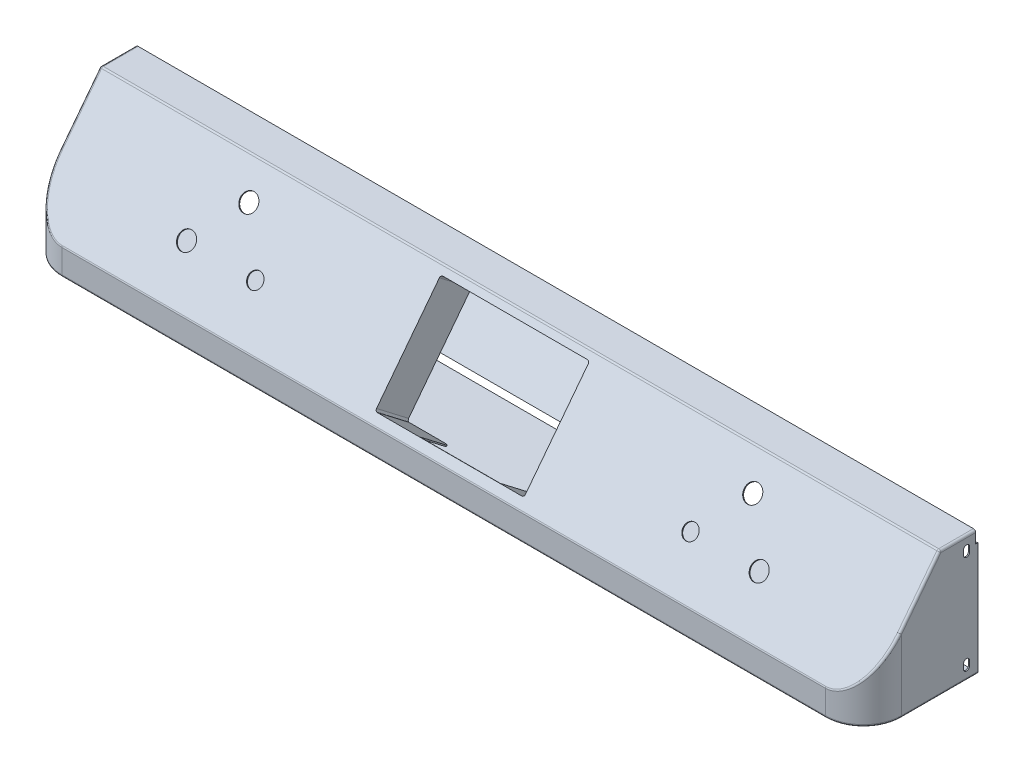
from build123d import *

# Parameters (mm, degrees)
SKETCH_1_W            = 1100
SKETCH_1_H            = 150
EXTRUDE_1_DEPTH       = 165
CUT_EXTRUDE_8_DEPTH   = 1115.831825882
FILLET_2_R            = 50
SHELL_1_T             = -1.5
HOLE_WIZARD_8_0_8_1_D = 8
SKETCH_20_W           = 83.034991693
SKETCH_20_H           = 41.985572191
CUT_EXTRUDE_7_DEPTH   = 1115.831825882
FILLET_5_R            = 3
CUT_EXTRUDE_10_DEPTH  = 1115.831825988
CUT_EXTRUDE_11_DEPTH  = 10
EXTRUDE_2_DEPTH       = 51.5
EXTRUDE_3_DEPTH       = 1.5
SKETCH_27_W           = 130
SKETCH_27_H           = 54.986401043
CUT_EXTRUDE_12_DEPTH  = 1.5
MOVE_FACE_1_BY        = 25
FILLET_6_R            = 10
SKETCH_28_R           = 11.25
SKETCH_28_R_2         = 9.75
CUT_EXTRUDE_13_DEPTH  = 1.5


with BuildPart() as part:
    # 草图1 → 凸台-拉伸1 (new body)
    with BuildSketch(Plane(origin=(0, 0, 0), x_dir=(1, 0, 0), z_dir=(0, 1, 0))):
        Rectangle(SKETCH_1_W, SKETCH_1_H)
    extrude(amount=EXTRUDE_1_DEPTH)

    # 草图21 → 切除-拉伸8 (cut, through all)
    with BuildSketch(Plane.ZY.offset(550)):
        Polygon((-25, 165), (75, 35), (149.01608628, 35), (149.01608628, 165), align=None)
    extrude(amount=-CUT_EXTRUDE_8_DEPTH, mode=Mode.SUBTRACT)

    # 圆角2
    fillet_2_edges = [part.edges().sort_by_distance(p)[0] for p in [
        (550, 17.5, 75),
        (-550, 17.5, 75),
    ]]
    fillet(fillet_2_edges, radius=FILLET_2_R)

    # 抽壳1
    shell_1_openings = [part.faces().sort_by_distance(p)[0] for p in [
        (0, 82.5, -75),
    ]]
    offset(amount=SHELL_1_T, openings=shell_1_openings, kind=Kind.INTERSECTION)

    # Ø8.0 (8) 直径孔1 (through all)
    with Locations(Plane.ZY.offset(550)):
        with Locations((-60, 147), (-60, 18)):
            Hole(HOLE_WIZARD_8_0_8_1_D / 2)

    # 草图20 → 切除-拉伸7 (cut, through all)
    with BuildSketch(Plane.ZY.offset(550)):
        with Locations((-113.517495847, 169.992786096)):
            Rectangle(SKETCH_20_W, SKETCH_20_H)
    extrude(amount=-CUT_EXTRUDE_7_DEPTH, mode=Mode.SUBTRACT)

    # 圆角5
    fillet_5_edges = [part.edges().sort_by_distance(p)[0] for p in [
        (550, 165, -48.5),
        (0, 165, -25),
        (-550, 132.5, 0),
        (550, 132.5, 0),
        (550, 0, -25),
        (0, 0, 75),
        (-535.355339059, 0, 60.355339059),
        (535.355339059, 0, 60.355339059),
        (0, 35, 75),
        (-539.140260323, 59.552655996, 56.113341541),
        (539.140260323, 59.552655996, 56.113341541),
        (-550, 0, -25),
        (-550, 165, -48.5),
    ]]
    fillet(fillet_5_edges, radius=FILLET_5_R)

    # 草图23 → 切除-拉伸10 (cut, through all)
    with BuildSketch(Plane(origin=(550, 0, 0), x_dir=(0, 0, -1), z_dir=(1, 0, 0))):
        with BuildLine():
            Line((64, 150), (64, 144))
            ThreePointArc((64, 144), (60, 140), (56, 144))
            Line((56, 144), (56, 150))
            ThreePointArc((56, 150), (60, 154), (64, 150))
        make_face()
        with BuildLine():
            Line((56, 15), (56, 21))
            ThreePointArc((56, 21), (60, 25), (64, 21))
            Line((64, 21), (64, 15))
            ThreePointArc((64, 15), (60, 11), (56, 15))
        make_face()
    extrude(amount=-CUT_EXTRUDE_10_DEPTH, mode=Mode.SUBTRACT)

    # 草图24 → 切除-拉伸11 (cut)
    with BuildSketch(Plane(origin=(0, 49.256505576, 64.033457249), x_dir=(1, 0, 0), z_dir=(0, 0.6097107608496924, 0.7926239891046002))):
        with BuildLine():
            Line((-94.5, 136), (94.5, 136))
            ThreePointArc((94.5, 136), (96.621320344, 135.121320344), (97.5, 133))
            Line((97.5, 133), (97.5, -2))
            ThreePointArc((97.5, -2), (96.621320344, -4.121320344), (94.5, -5))
            Line((94.5, -5), (-94.5, -5))
            ThreePointArc((-94.5, -5), (-96.621320344, -4.121320344), (-97.5, -2))
            Line((-97.5, -2), (-97.5, 133))
            ThreePointArc((-97.5, 133), (-96.621320344, 135.121320344), (-94.5, 136))
        make_face()
    extrude(amount=-CUT_EXTRUDE_11_DEPTH, mode=Mode.SUBTRACT)

    # 草图25 → 凸台-拉伸2 (add)
    with BuildSketch(Plane(origin=(0, 48.341939435, 62.844521265), x_dir=(-1, 0, 0), z_dir=(0, -0.6097107608496924, -0.7926239891046002))):
        with BuildLine():
            Line((99, -2), (99, 133))
            ThreePointArc((99, 133), (97.681980515, 136.181980515), (94.5, 137.5))
            Line((94.5, 137.5), (-94.5, 137.5))
            ThreePointArc((-94.5, 137.5), (-97.681980515, 136.181980515), (-99, 133))
            Line((-99, 133), (-99, -2))
            ThreePointArc((-99, -2), (-97.681980515, -5.181980515), (-94.5, -6.5))
            Line((-94.5, -6.5), (94.5, -6.5))
            ThreePointArc((94.5, -6.5), (97.681980515, -5.181980515), (99, -2))
        make_face()
        with BuildLine():
            Line((94.5, 136), (-94.5, 136))
            ThreePointArc((-94.5, 136), (-96.621320344, 135.121320344), (-97.5, 133))
            Line((-97.5, 133), (-97.5, -2))
            ThreePointArc((-97.5, -2), (-96.621320344, -4.121320344), (-94.5, -5))
            Line((-94.5, -5), (94.5, -5))
            ThreePointArc((94.5, -5), (96.621320344, -4.121320344), (97.5, -2))
            Line((97.5, -2), (97.5, 133))
            ThreePointArc((97.5, 133), (96.621320344, 135.121320344), (94.5, 136))
        make_face(mode=Mode.SUBTRACT)
    extrude(amount=EXTRUDE_2_DEPTH)

    # 草图26 → 凸台-拉伸3 (add)
    with BuildSketch(Plane(origin=(0, 16.941835251, 22.024385827), x_dir=(-1, 0, 0), z_dir=(0, -0.6097107608496924, -0.7926239891046002))):
        with BuildLine():
            Line((-99, 66), (99, 66))
            Line((99, 66), (99, 133))
            ThreePointArc((99, 133), (97.681980515, 136.181980515), (94.5, 137.5))
            Line((94.5, 137.5), (-94.5, 137.5))
            ThreePointArc((-94.5, 137.5), (-97.681980515, 136.181980515), (-99, 133))
            Line((-99, 133), (-99, 66))
        make_face()
    extrude(amount=EXTRUDE_3_DEPTH)

    # 草图27 → 切除-拉伸12 (cut)
    with BuildSketch(Plane(origin=(0, -3.963119946, 3.048553804), x_dir=(1, 0, 0), z_dir=(0, 0.7926239891046, -0.6097107608496924))):
        with Locations((0, -51.793475292)):
            Rectangle(SKETCH_27_W, SKETCH_27_H)
    extrude(amount=-CUT_EXTRUDE_12_DEPTH, mode=Mode.SUBTRACT)

    # Move Face 1: a face moved outward by 25.0
    extrude(part.faces().sort_by_distance((-65, 28.084299406, 45.940290421))[0], amount=MOVE_FACE_1_BY, dir=(1, 0, 0))

    # 圆角6
    fillet_6_edges = [part.edges().sort_by_distance(p)[0] for p in [
        (65, 12.384247314, 25.530222701),
        (-40, 12.384247314, 25.530222701),
    ]]
    fillet(fillet_6_edges, radius=FILLET_6_R)

    # 草图28 → 切除-拉伸13 (cut)
    with BuildSketch(Plane(origin=(0, 49.256505576, 64.033457249), x_dir=(1, 0, 0), z_dir=(0, 0.6097107608496924, 0.7926239891046))):
        with Locations(Location((-330, 105, 0), (0, 0, 270))):
            Circle(SKETCH_28_R)
        with Locations(Location((330, 105, 0), (0, 0, 270))):
            Circle(SKETCH_28_R)
        with Locations(Location((375, 45, 0), (0, 0, 270))):
            Circle(SKETCH_28_R)
        with Locations(Location((285, 45, 0), (0, 0, 270))):
            Circle(SKETCH_28_R_2)
        with Locations(Location((-285, 45, 0), (0, 0, 270))):
            Circle(SKETCH_28_R_2)
        with Locations(Location((-375, 45, 0), (0, 0, 270))):
            Circle(SKETCH_28_R)
    extrude(amount=-CUT_EXTRUDE_13_DEPTH, mode=Mode.SUBTRACT)


solid = part.part
